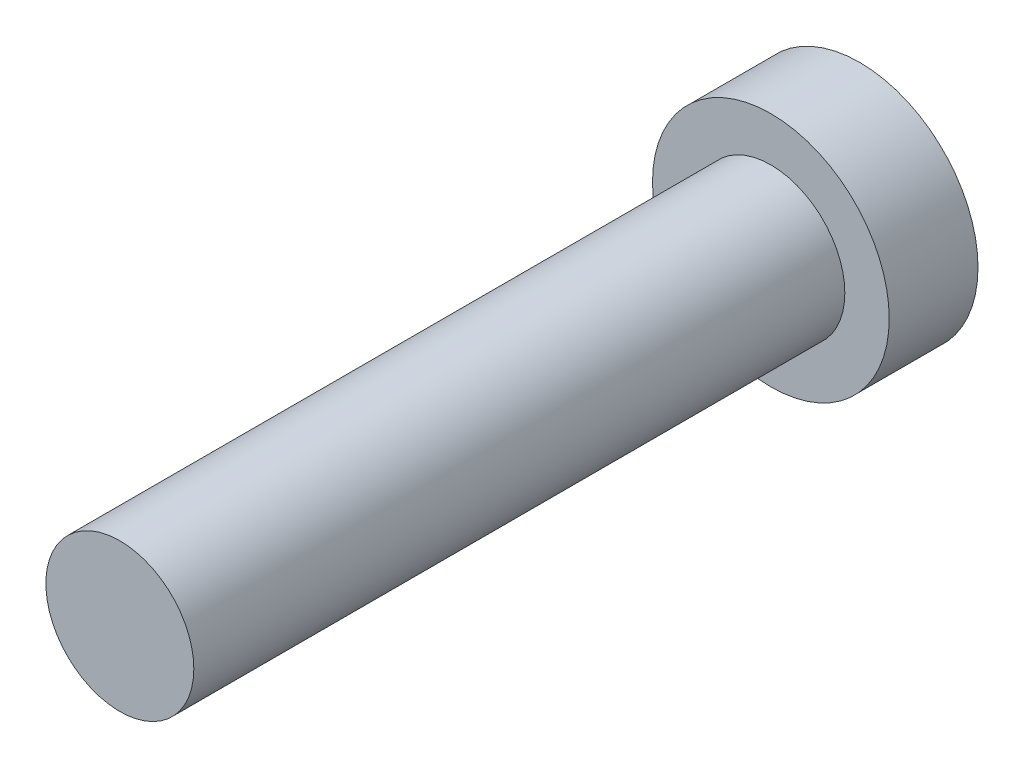
SolidWorks part; units mm, degrees
ref_plane "Front Plane" through (0, 0, 0) normal (0, 0, 1) x (1, 0, 0)
ref_plane "Top Plane" through (0, 0, 0) normal (0, 1, 0) x (1, 0, 0)
ref_plane "Right Plane" through (0, 0, 0) normal (1, 0, 0) x (0, 0, -1)
sketch "Sketch1" plane through (0, 0, 0) normal (0, 0, 1) x (1, 0, 0)
  circle A0 centre (0, 0) radius 25
  dimension "D1" = 50
extrude "Boss-Extrude1" add sketch "Sketch1" against normal blind 220
cosmetic thread "Cosmetic Thread1" parameters "D2"=18.631
sketch "Sketch2" plane through (0, 0, -220) normal (0, 0, -1) x (-1, 0, 0)
  circle A0 centre (0, 0) radius 40
  dimension "D1" = 80
extrude "Boss-Extrude2" add sketch "Sketch2" along normal blind 30
